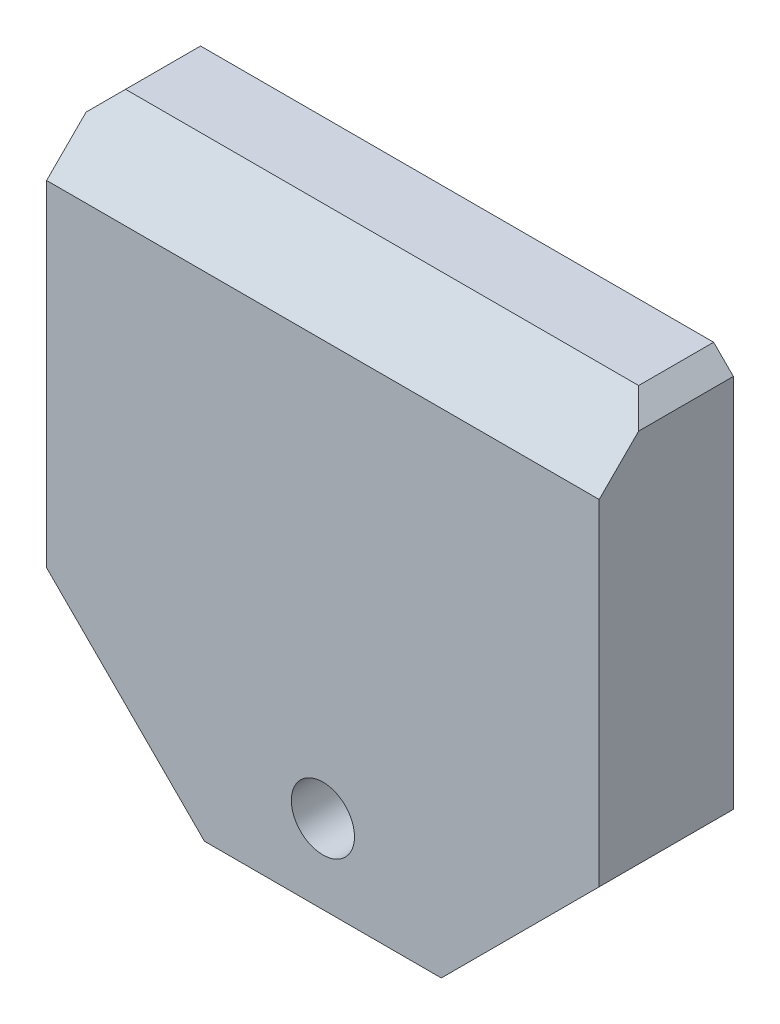
from build123d import *

# Parameters (mm, degrees)
SKETCH1_W           = 140
SKETCH1_H           = 140
BOSS_EXTRUDE1_DEPTH = 34
SKETCH3_R           = 8
CUT_EXTRUDE3_DEPTH  = 105.670912865
CHAMFER1_SIZE       = 5
CHAMFER2_SIZE       = 15
CHAMFER3_SIZE       = 40


with BuildPart() as part:
    # Sketch1 → Boss-Extrude1 (new body)
    with BuildSketch(Plane.XY):
        Rectangle(SKETCH1_W, SKETCH1_H)
    extrude(amount=BOSS_EXTRUDE1_DEPTH)

    # Sketch3 → Cut-Extrude3 (cut, through all)
    with BuildSketch(Plane.XY.offset(34)):
        with Locations((0, -50)):
            Circle(SKETCH3_R)
    extrude(amount=-CUT_EXTRUDE3_DEPTH, mode=Mode.SUBTRACT)

    # Chamfer1
    chamfer1_edges = [part.edges().sort_by_distance(p)[0] for p in [
        (-70, 70, 17),
        (70, 70, 17),
    ]]
    chamfer(chamfer1_edges, length=CHAMFER1_SIZE)

    # Chamfer2
    chamfer2_edges = [part.edges().sort_by_distance(p)[0] for p in [
        (0, 70, 34),
    ]]
    chamfer(chamfer2_edges, length=CHAMFER2_SIZE)

    # Chamfer3
    chamfer3_edges = [part.edges().sort_by_distance(p)[0] for p in [
        (70, -70, 17),
        (-70, -70, 17),
    ]]
    chamfer(chamfer3_edges, length=CHAMFER3_SIZE)


solid = part.part
